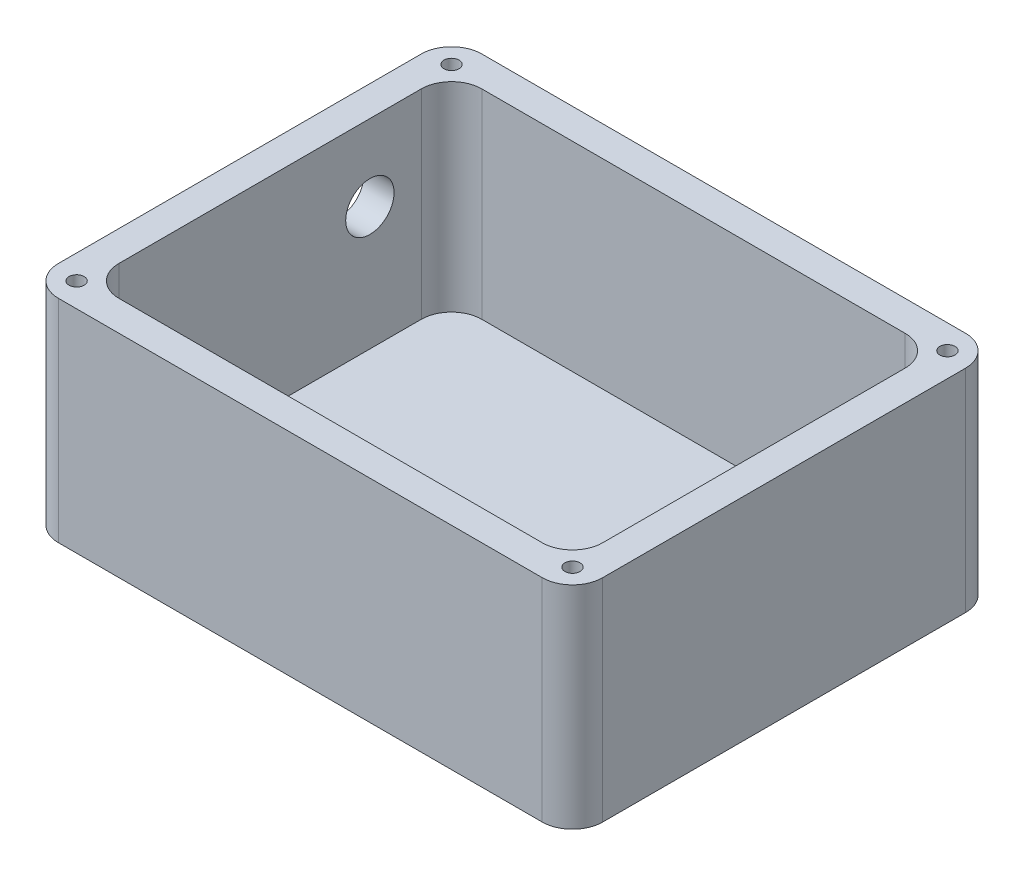
SolidWorks part; units mm, degrees
ref_plane "Front Plane" through (0, 0, 0) normal (0, 0, 1) x (1, 0, 0)
ref_plane "Top Plane" through (0, 0, 0) normal (0, 1, 0) x (1, 0, 0)
ref_plane "Right Plane" through (0, 0, 0) normal (1, 0, 0) x (0, 0, -1)
sketch "Sketch1" plane through (0, 0, 0) normal (0, 1, 0) x (1, 0, 0)
  line L1 (-45, -35) -> (45, -35)
  line L2 (-45, -35) -> (-45, 35)
  line L3 (-45, 35) -> (45, 35)
  line L4 (45, -35) -> (45, 35)
  line L5 (-45, -35) -> (45, 35) construction
  line L6 (-45, 35) -> (45, -35) construction
  point P0 (0, 0)
  dimension "D1" = 90
  dimension "D2" = 70
extrude "Boss-Extrude1" add sketch "Sketch1" along normal blind 35
sketch "Sketch2" plane through (0, 35, 0) normal (0, 1, 0) x (1, 0, 0)
  line L1 (-40, -30) -> (40, -30)
  line L2 (-40, -30) -> (-40, 30)
  line L3 (-40, 30) -> (40, 30)
  line L4 (40, -30) -> (40, 30)
  line L5 (-40, -30) -> (40, 30) construction
  line L6 (-40, 30) -> (40, -30) construction
  point P0 (0, 0)
  dimension "D1" = 80
  dimension "D2" = 60
extrude "Cut-Extrude1" cut sketch "Sketch2" against normal blind 33
fillet "Fillet1" radius 5 8 edges at (45, 17.5, -35) (45, 17.5, 35) (-45, 17.5, 35) (-45, 17.5, -35) (-40, 18.5, 30) (40, 18.5, 30) (40, 18.5, -30) (-40, 18.5, -30)
hole_wizard "M3 Tapped Hole1" positions "Sketch4" profile "Sketch6" tap size "M3" standard "GB"
sketch "Sketch4" plane through (0, 35, 0) normal (0, 1, 0) x (1, 0, 0)
  line L0 (40, 35) -> (-40, 35) construction
  line L1 (-45, 30) -> (-45, -30) construction
  line L2 (45, -30) -> (45, 30) construction
  line L3 (-40, -35) -> (40, -35) construction
  point P0 (-41, 31)
  point P2 (41, 31)
  point P4 (41, -31)
  point P6 (-41, -31)
  dimension "D1" = 4
  dimension "D2" = 4
  dimension "D3" = 4
  dimension "D4" = 4
  dimension "D5" = 4
  dimension "D6" = 4
  dimension "D7" = 4
  dimension "D8" = 4
sketch "Sketch6" plane through (-41, 35, -31) normal (1, 0, 0) x (0, 0, 1)
  line L0 (0, 0) -> (0, 9.2511)
  line L1 (0, 9.2511) -> (1.25, 8.5)
  line L2 (1.25, 8.5) -> (1.25, 0)
  line L5 (1.25, 0) -> (0, 0)
  line L10 (0, 9.2511) -> (-1.25, 8.5) construction
  line L11 (0, -6.35) -> (0, 107.95) construction
  dimension "螺纹孔钻头直径" = 2.5
  dimension "螺纹孔钻头深度" = 8.5
  dimension "导头角度" = 118
cosmetic thread "Cosmetic thread 1" parameters "D1"=6, "D2"=3
cosmetic thread "Cosmetic thread 2" parameters "D1"=6, "D2"=3
cosmetic thread "Cosmetic thread 3" parameters "D1"=6, "D2"=3
cosmetic thread "Cosmetic thread 4" parameters "D1"=6, "D2"=3
sketch "Sketch7" plane through (-45, 0, 0) normal (-1, 0, 0) x (0, 0, 1)
  line L0 (-30, 0) -> (30, 0) construction
  line L1 (-35, 0) -> (-35, 35) construction
  circle A0 centre (-16.5, 22.4) radius 4
  dimension "D1" = 8
  dimension "D2" = 22.4
  dimension "D3" = 18.5
extrude "Cut-Extrude2" cut sketch "Sketch7" against normal blind 10
